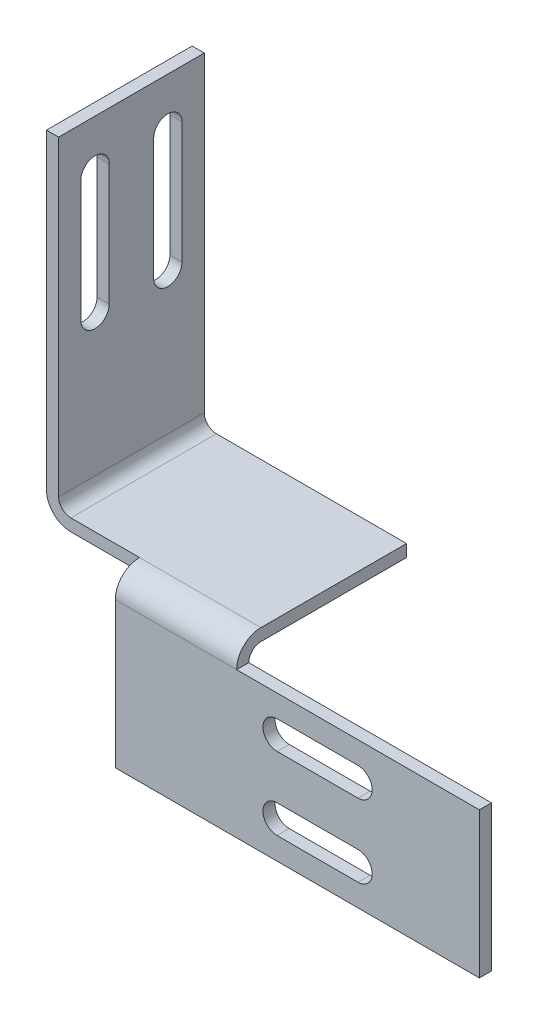
SolidWorks part; units mm, degrees
ref_plane "Front Plane" through (0, 0, 0) normal (0, 0, 1) x (1, 0, 0)
ref_plane "Top Plane" through (0, 0, 0) normal (0, 1, 0) x (1, 0, 0)
ref_plane "Right Plane" through (0, 0, 0) normal (1, 0, 0) x (0, 0, -1)
sketch "Sketch1" plane through (0, 0, 0) normal (0, 0, 1) x (1, 0, 0)
  line L0 (0, 0) -> (0, 40)
  line L1 (0, 0) -> (25, 0)
  dimension "D1" = 25
  dimension "D2" = 40
extrude "Extrude-Thin1" add sketch "Sketch1" along normal blind 18 thin thin type one direction wall 1.5
fillet "Fillet2" radius 1.5 1 edges at (0, 0, 9)
fillet "Fillet3" radius 3 1 edges at (-1.5, -1.5, 9)
sketch "Sketch4" plane through (25, 0, 0) normal (1, 0, 0) x (0, 0, -1)
  line L2 (-21, -3) -> (-21, -21)
  line L3 (-21, -21) -> (-19.5, -21)
  line L4 (-19.5, -3) -> (-19.5, -21)
  line L5 (-18, 0) -> (-18, -1.5) construction
  line L6 (-18, 0) -> (-18, -1.5)
  arc A0 (-18, -1.5) -> (-19.5, -3) centre (-18, -3) ccw
  arc A1 (-18, 0) -> (-21, -3) centre (-18, -3) ccw
  dimension "D3" = 3
  dimension "D4" = 6
  dimension "D1" = 1.5
  dimension "D2" = 18
extrude "Boss-Extrude1" add sketch "Sketch4" along normal blind 30 and the other way blind 15
sketch "Sketch5" plane through (55, 0, 0) normal (1, 0, 0) x (0, 0, -1)
  line L1 (-21, -3) -> (-18, -3)
  line L2 (-21, -3) -> (-21, 0)
  line L3 (-21, 0) -> (-18, 0)
  line L4 (-18, -3) -> (-18, 0)
extrude "Cut-Extrude2" cut sketch "Sketch5" against normal up to surface (30 mm away) up to face at (25, -0.5625, 13.5)
sketch "Sketch6" plane through (-1.5, 0, 0) normal (-1, 0, 0) x (0, 0, 1)
  line L0 (4.5, 34) -> (4.5, 19) construction
  line L1 (6.25, 34) -> (6.25, 19)
  line L2 (2.75, 34) -> (2.75, 19)
  line L3 (9, 40) -> (9, 8.6298) construction
  line L4 (18, 40) -> (0, 40) construction
  line L5 (13.5, 34) -> (13.5, 19) construction
  line L6 (11.75, 34) -> (11.75, 19)
  line L7 (15.25, 34) -> (15.25, 19)
  arc A0 (6.25, 34) -> (2.75, 34) centre (4.5, 34) ccw
  arc A1 (2.75, 19) -> (6.25, 19) centre (4.5, 19) ccw
  arc A2 (11.75, 34) -> (15.25, 34) centre (13.5, 34) cw
  arc A3 (15.25, 19) -> (11.75, 19) centre (13.5, 19) cw
  point P2 (4.5, 26.5)
  point P13 (13.5, 26.5)
  dimension "D1" = 1.75
  dimension "D3" = 9
  dimension "D4" = 6
  dimension "D2" = 15
extrude "Cut-Extrude3" cut sketch "Sketch6" against normal through all
sketch "Sketch7" plane through (0, 0, 21) normal (0, 0, 1) x (1, 0, 0)
  line L0 (30, -7.5) -> (40, -7.5) construction
  line L1 (30, -5.75) -> (40, -5.75)
  line L2 (30, -9.25) -> (40, -9.25)
  line L3 (55, -12) -> (10, -12) construction
  line L4 (55, -3) -> (55, -21) construction
  line L5 (10, -3) -> (10, -21) construction
  line L6 (30, -16.5) -> (40, -16.5) construction
  line L7 (30, -18.25) -> (40, -18.25)
  line L8 (30, -14.75) -> (40, -14.75)
  arc A0 (30, -5.75) -> (30, -9.25) centre (30, -7.5) ccw
  arc A1 (40, -9.25) -> (40, -5.75) centre (40, -7.5) ccw
  arc A2 (30, -18.25) -> (30, -14.75) centre (30, -16.5) cw
  arc A3 (40, -14.75) -> (40, -18.25) centre (40, -16.5) cw
  point P2 (35, -7.5)
  point P15 (35, -16.5)
  dimension "D1" = 1.75
  dimension "D3" = 9
  dimension "D4" = 15
  dimension "D2" = 10
extrude "Cut-Extrude4" cut sketch "Sketch7" against normal blind 10
